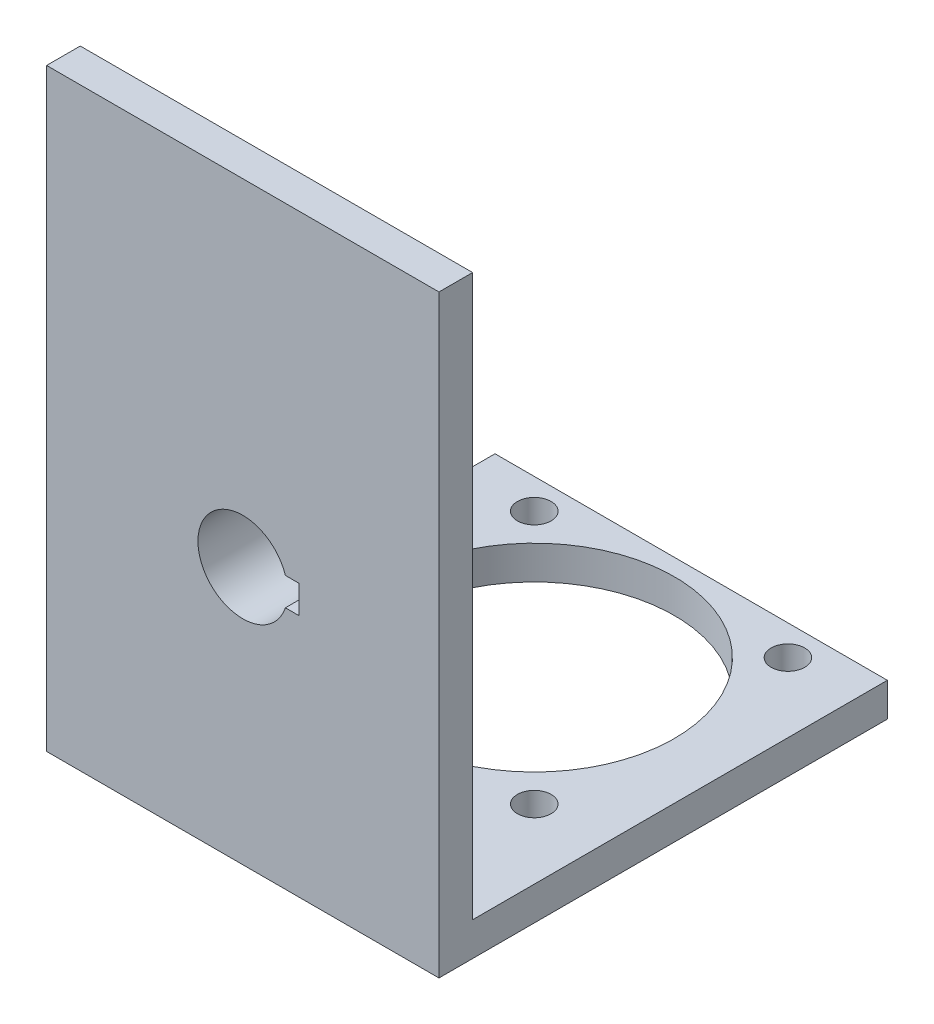
SolidWorks part; units mm, degrees
ref_plane "Front Plane" through (0, 0, 0) normal (0, 0, 1) x (1, 0, 0)
ref_plane "Top Plane" through (0, 0, 0) normal (0, 1, 0) x (1, 0, 0)
ref_plane "Right Plane" through (0, 0, 0) normal (1, 0, 0) x (0, 0, -1)
sketch "Sketch1" plane through (0, 0, 0) normal (0, 0, 1) x (1, 0, 0)
  line L1 (-35, 60) -> (35, 60)
  line L2 (-35, 60) -> (-35, -40)
  line L3 (-35, -40) -> (35, -40)
  line L4 (35, 60) -> (35, -40)
  circle A0 centre (0, 0) radius 8
  dimension "D1" = 16
  dimension "D2" = 70
  dimension "D3" = 35
  dimension "D4" = 40
  dimension "D5" = 100
extrude "Boss-Extrude1" add sketch "Sketch1" along normal blind 6
sketch "Sketch2" plane through (0, 0, 0) normal (0, 0, -1) x (-1, 0, 0)
  circle A0 centre (0, 0) radius 8 construction
  circle A1 centre (0, 0) radius 8
  circle A2 centre (0, 0) radius 18
  dimension "D1" = 10
extrude "Boss-Extrude2" add sketch "Sketch2" along normal blind 10
sketch "Sketch3" plane through (0, -40, 0) normal (0, -1, 0) x (1, 0, 0)
  line L0 (-35, 6) -> (35, 6)
  line L1 (-35, 6) -> (-35, -74)
  line L2 (35, 6) -> (35, -74)
  line L3 (-35, -74) -> (35, -74)
  dimension "D1" = 80
extrude "Boss-Extrude3" add sketch "Sketch3" along normal blind 6
sketch "Sketch4" plane through (0, 0, -10) normal (0, 0, -1) x (-1, 0, 0)
  line L1 (-10, 2.5) -> (-5.071, 2.5)
  line L2 (-10, 2.5) -> (-10, -2.5)
  line L3 (-10, -2.5) -> (-5.071, -2.5)
  line L4 (-5.071, 2.5) -> (-5.071, -2.5)
  dimension "D1" = 5
  dimension "D2" = 2.5
  dimension "D3" = 10
extrude "Cut-Extrude1" cut sketch "Sketch4" against normal through all
sketch "Sketch5" plane through (0, -40, 0) normal (0, 1, 0) x (1, 0, 0)
  circle A0 centre (-22.6274, 68.6274) radius 3.0065
  circle A1 centre (22.6274, 68.6274) radius 3
  circle A2 centre (22.6274, 23.3726) radius 3
  circle A3 centre (-22.6274, 23.3726) radius 3
  circle A4 centre (-0.0091, 46) radius 25.0091
extrude "Cut-Extrude2" cut sketch "Sketch5" against normal blind 6
